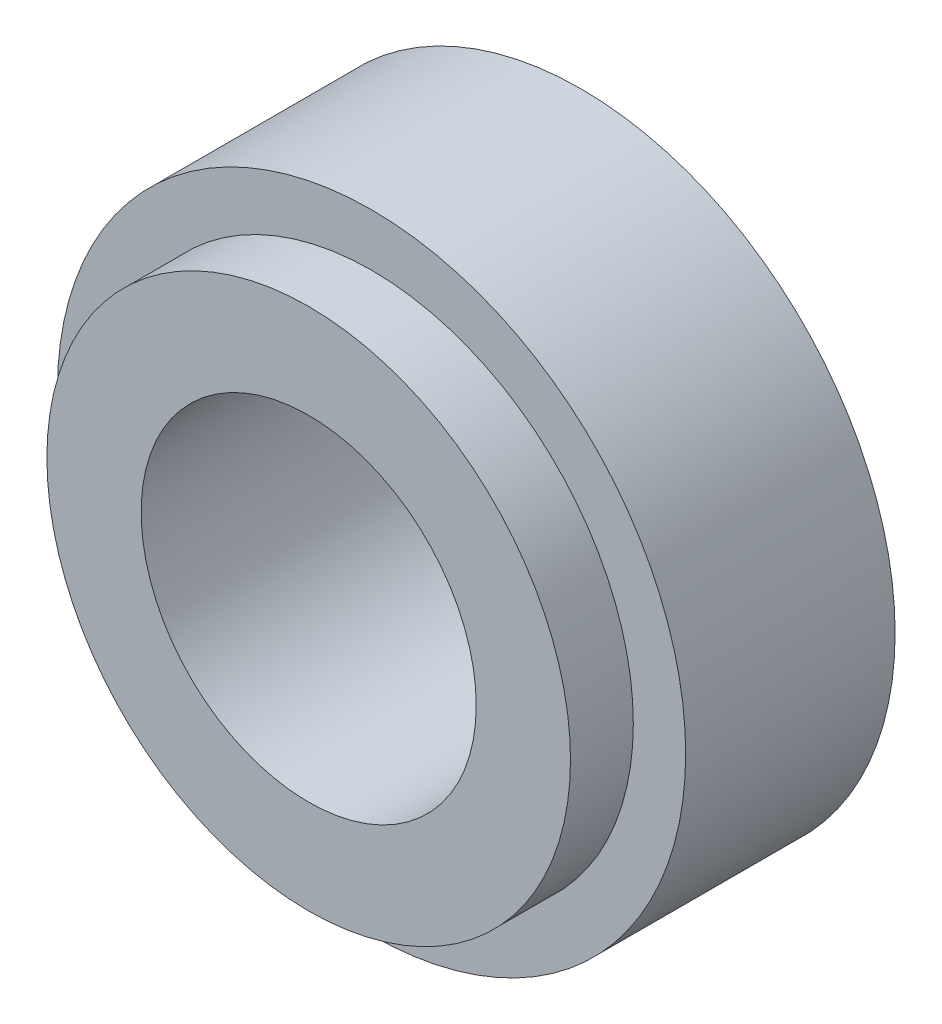
from build123d import *

# Parameters (mm, degrees)
SKETCH1_R           = 15
BOSS_EXTRUDE1_DEPTH = 10
SKETCH2_R           = 12.5
BOSS_EXTRUDE2_DEPTH = 3
SKETCH3_R           = 8
CUT_EXTRUDE1_DEPTH  = 25.879710609


with BuildPart() as part:
    # Sketch1 → Boss-Extrude1 (new body)
    with BuildSketch(Plane.XY):
        Circle(SKETCH1_R)
    extrude(amount=BOSS_EXTRUDE1_DEPTH)

    # Sketch2 → Boss-Extrude2 (add)
    with BuildSketch(Plane.XY.offset(10)):
        Circle(SKETCH2_R)
    extrude(amount=BOSS_EXTRUDE2_DEPTH)

    # Sketch3 → Cut-Extrude1 (cut, through all)
    with BuildSketch(Plane.XY.offset(13)):
        Circle(SKETCH3_R)
    extrude(amount=-CUT_EXTRUDE1_DEPTH, mode=Mode.SUBTRACT)


solid = part.part
